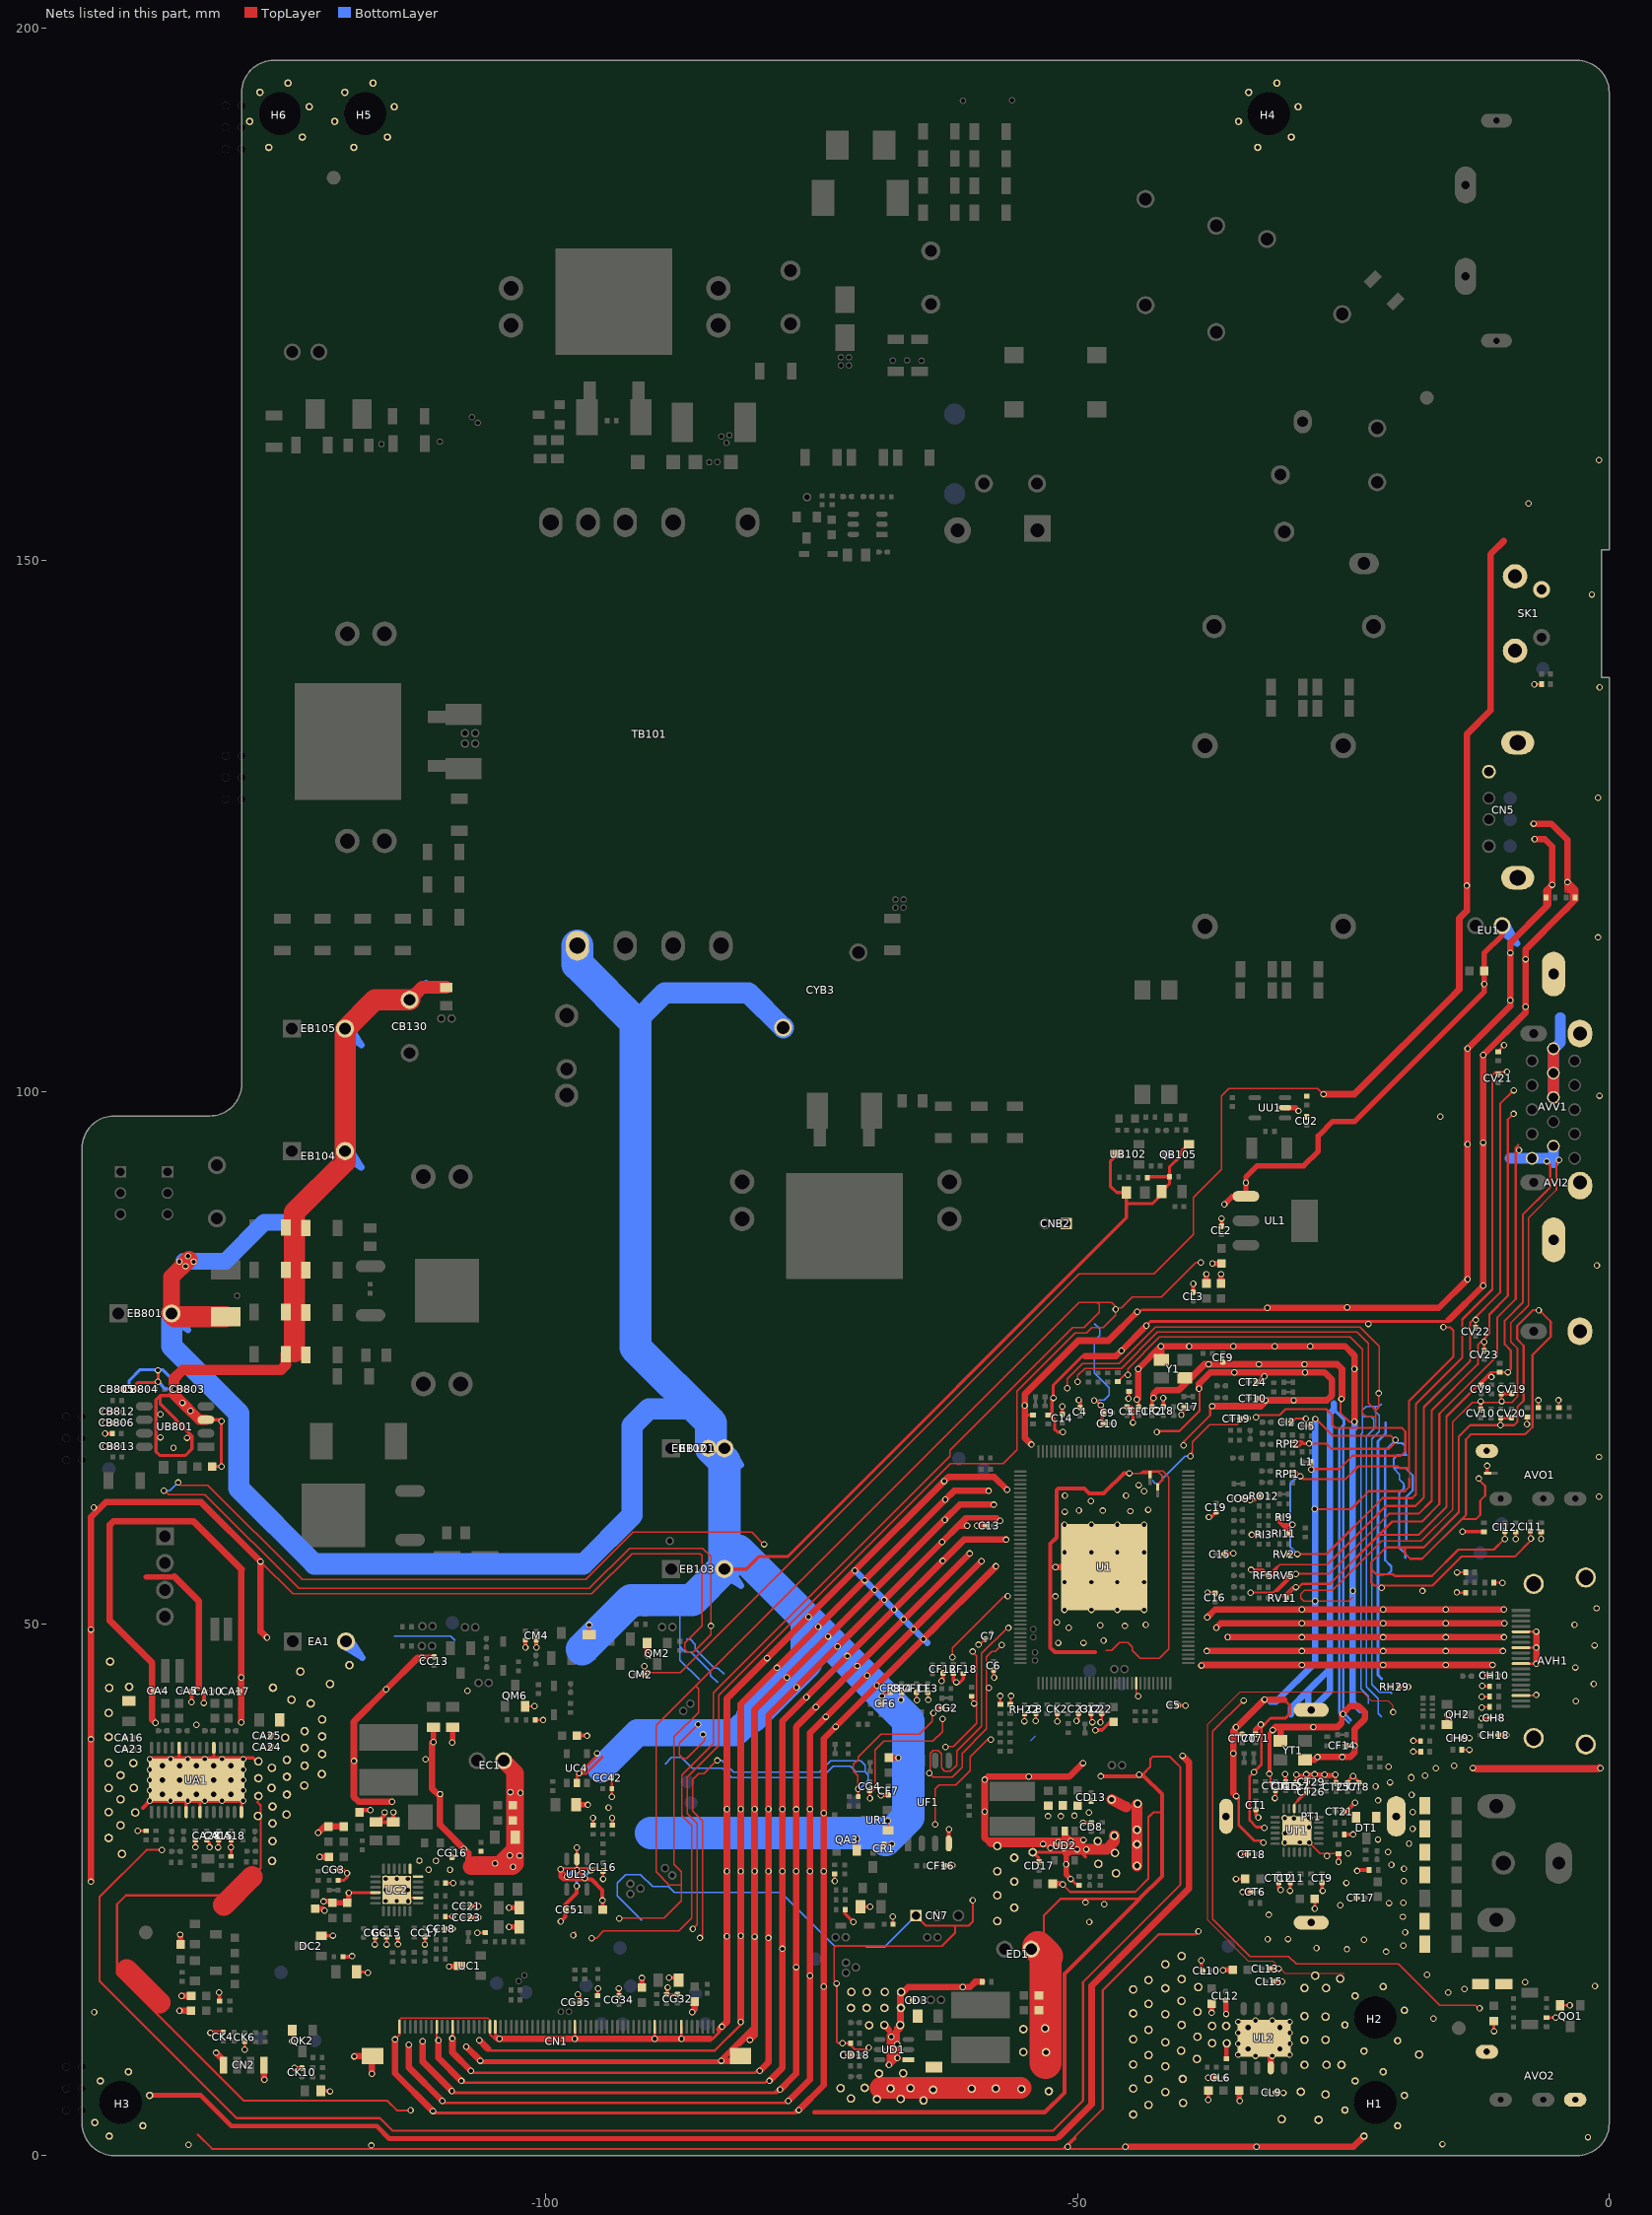
[diagram p0: the nets of this part, all layers, seen from the top]
# Altium PCB MISC86383-9.PcbDoc (part 10 of 18)
Units mm, origin at the board's own origin, x right, y up, seen from the top; angles counter-clockwise.
Board outline 143.6 x 197 mm, 2 copper layers (TopLayer, BottomLayer), stack 1.571 mm thick; 743 components, 401 nets, 2996 pads, 1077 vias.
Unrouted connection lines stored in the file: 4.

## Via types
v1: diameter 0.6, hole 0.4, TopLayer to BottomLayer, tented both sides, 993 vias
v2: diameter 0.6, hole 0.4, TopLayer to BottomLayer, 65 vias
v3: diameter 0.7, hole 0.5, TopLayer to BottomLayer, tented both sides, 15 vias
v4: diameter 0.8, hole 0.5, TopLayer to BottomLayer, tented both sides, 4 vias

## Nets (pads, with @x,y where several pads share a name; then routed paths per layer and width w, separated by ;. In a path a pad name is that pad's centre, name@x,y a point inside that pad or via, vN(x,y) a via of type N, cw(c..) or ccw(c..) an arc to the next point about the centre after c; other vN are vias at no path point) (continued)
GND: (continued)
  TopLayer w0.203: v1(-138.372,30.534) RA1.1@-137.578,30.534 ; v1(-136.105,28.735) -137.55,28.735 -141.962,24.323 -141.962,16.383 -129.084,3.505 ; RA14.1@-132.947,29.659 -132.947,29.053 -132.939,29.046 v1(-132.939,28.981) ; -132.715,1.956 -131.386,0.627 -51.386,0.627 ; -128.321,3.505 -129.084,3.505 ; CK6.1@-128.321,10.7 -128.321,9.97 v1(-128.308,9.957) ; -127.114,33.223 -126.809,32.918 -126.809,27.026 -129.375,24.46 -139.49,24.46 -140.311,23.639 -140.311,17.067 -128.4,5.156 -114.912,5.156 -113.998,4.242 v1(-112.712,4.242) ; v1(-114.173,10.909) -113.75,11.332 CN1.1@-113.75,12.103 ; CN1.8@-110.25,12.103 -110.25,10.987 v1(-110.084,10.82) ; v1@-108.75,10.808 CN1.11@-108.75,12.103 ; v1(-106.426,20.93) -106.426,20.98 -106.394,20.948 RC3.1@-105.715,20.948 ; CN1.18@-105.25,12.103 -105.25,11.398 -104.825,10.973 ; CN1.19@-104.75,12.103 -104.75,11.38 v1(-104.343,10.973) ; QM6.E@-101.943,42.228 -101.105,42.228 v1(-101.067,42.266) ; RM10.2@-100.997,40.957 -100.266,40.957 v1(-100.254,40.945) ; v1(-97.422,20.697) -97.235,20.884 -97.235,20.996 ; v1(-97.282,10.973) -97.25,11.005 CN1.34@-97.25,12.103 ; RG12.1@-95.123,15.024 -95.123,15.672 -95.098,15.697 v1(-95.098,15.71) ; v1(-89.764,10.973) -89.75,10.986 CN1.49@-89.75,12.103 ; CN1.54@-87.25,12.103 -87.25,10.987 v1(-87.236,10.973) ; RA38.1@-72.83,26.484 -72.83,25.87 -72.819,25.859 v1(-72.819,25.807) ; v1(-72.649,16.186) -72.644,16.181 -72.644,10.693 -72.517,10.566 v1(-72.085,10.566) -72.079,10.56 RD5.1@-71.343,10.56 -71.343,10.383 -70.942,9.982 -69.748,9.982 -69.596,10.135 v1(-69.621,10.135) ; v1(-72.034,9.449) -72.009,9.449 -72.007,9.451 CD18.1@-71.345,9.451 ; QA3.E@-70.744,28.713 -70.744,29.767 v1(-70.731,29.78) ; v1(-70.637,34.468) -70.637,34.315 -70.619,34.297 RR2.2@-70.619,33.757 ; CG4.2@-69.545,34.297 -69.545,33.63 v1(-69.52,33.604) ; CF6.2@-68.472,42.469 -68.472,43.11 v1(-68.377,43.205) -68.065,43.517 CF8.2@-67.615,43.517 ; CR1.1@-68.191,29.291 -68.184,29.298 v1(-67.454,29.298) ; v1(-67.835,31.457) -67.81,31.431 UR1.1@-67.81,30.58 ; v1(-67.359,22.456) -67.359,22.413 -67.334,22.388 RA31.1@-67.334,21.754 ; v1(-66.598,42.839) -66.562,42.875 -66.548,42.875 CF4.2@-66.548,43.517 ; CN7.1@-65.195,22.555 -64.255,21.615 -61.493,21.615 ; CF11.2@-65.151,43.517 -65.151,42.875 v1(-65.1,42.824) ; CF3.2@-64.069,43.521 -64.069,43.008 -64.042,42.981 v1(-64.042,42.844) ; v1@-63.599,41.607 -63.094,42.113 CG2.2@-62.782,42.113 ; -62.743,19.71 -61.493,20.96 -61.493,21.615 ; DR1.A@-59.957,43.187 -59.957,42.939 -59.703,42.685 -59.703,42.52 v1(-59.715,42.507) ; v1(-59.842,24.003) -59.842,21.996 -60.223,21.615 -61.493,21.615 ; v1(-59.294,48.036) -59.396,48.137 -59.091,48.137 C7.1@-58.68,48.548 ; DV2.A@-57.262,42.415 v1(-57.262,43.21) ; DV1.A@-56.297,42.415 -56.297,43.159 v1(-56.246,43.21) ; v1(-54.988,40.837) -54.988,40.899 -54.976,40.912 RH22.1@-54.976,41.515 ; ED1.2@-54.351,19.406 -53.162,20.594 -53.162,22.552 -51.585,24.13 -44.181,24.13 -44.162,24.149 ; v1(-53.934,40.875) -53.91,40.9 -53.91,41.002 C8.1@-53.91,41.553 C8.1@-53.91,41.728 ; v1(-51.903,40.835) CK2.2@-51.903,41.553 ; v1(-51.384,25.476) -50.698,24.79 -44.581,24.79 -43.332,26.039 -43.332,31.801 -42.875,32.258 -42.056,32.258 ; v1@-51.013,0.789 v1@-50.981,0.821 ; v1(-50.911,0.821) v1@-50.981,0.821 ; DT3.A@-46.215,72.765 -45.587,73.393 v1(-45.263,73.393) ; v1(-45.494,0.826) -45.693,0.627 -51.386,0.627 ; v1@-44.226,35.839 v1(-44.194,35.808) ; -44.028,64.152 -43.86,64.321 -43.307,64.321 -42.443,64.321 -42.021,63.899 -42.021,63.516 -42.021,63.482 RA2.JP_2K@-42.456,63.047 ; -43.891,35.801 -43.147,36.545 -43.147,37.281 -42.933,37.495 -41.305,37.495 -40.594,36.784 ; v1(-42.543,68.038) -42.467,68.114 -40.421,68.114 -38.521,70.014 ; -40.967,37.158 -40.316,36.507 -40.316,25.469 -49.484,16.301 -49.484,5.15 -52.306,2.329 -114.42,2.329 -115.596,3.505 -129.084,3.505 ; v1(-40.029,66.781) -40.029,67.105 -37.53,69.604 -37.53,70.256 v1(-37.327,70.459) ; v1(-38.618,21.078) -38.893,20.803 -42.36,20.803 -47.63,15.533 -47.63,4.382 -50.228,1.784 ; v1(-38.568,72.115) -38.521,72.068 -38.521,70.014 ; -38.521,70.663 -38.521,70.014 ; CT19.1@-34.66,69.27 -34.601,69.329 v1(-33.982,69.329) ; v1(-33.733,52.928) -33.713,52.948 -31.587,52.948 -31.461,53.075 ; v1(-33.225,69.408) v1@-33.182,69.366 ; v1@-33.182,69.291 v1@-33.182,69.366 ; v2(-31.953,35.89) -31.858,35.795 -31.858,34.79 CT14.1@-31.379,34.311 ; -30.687,52.547 -29.791,53.444 v1(-29.462,53.444) v1@-29.498,53.407 ; RV11.1@-30.342,52.428 -30.342,52.564 v1@-29.498,53.407 ; RV5.1@-30.139,54.562 -30.139,54.397 -31.461,53.075 ; RV5.1@-30.136,54.683 -29.733,54.683 v1@-29.661,54.611 ; RV2.1@-30.136,56.512 -29.444,56.512 -29.307,56.649 v1(-29.307,56.552) -26.563,56.552 -21.305,61.811 ; CI2.1@-29.856,68.963 -29.517,69.302 v1@-28.53,69.302 ; RPI1.6@-29.797,63.849 -29.074,63.849 v1(-29.053,63.871) -28.794,63.612 -24.79,63.612 -23.594,64.808 -19.875,64.808 -19.71,64.643 -18.877,64.643 -18.826,64.694 ; v1@-29.589,53.407 v1@-29.498,53.407 ; v1@-29.447,54.689 -26.351,54.689 -20.697,60.343 -17.909,60.343 -16.698,61.554 -16.698,70.058 -12.344,74.411 -12.344,76.238 -11.273,77.309 -11.273,79.083 -9.522,80.834 -9.522,97.418 v1(-8.992,97.949) v1@-8.9,98.04 ; v1@-28.591,69.2 v1(-28.51,69.282) ; v1(-28.227,66.944) -26.6,66.944 -26.114,66.458 -20.714,66.458 -20.01,67.162 v1@-20.01,67.276 ; L1.1@-28.018,65.23 -28.024,65.224 v1@-28.024,64.544 ; CI5.1@-27.908,68.709 CI5.1@-28.022,68.595 -28.022,68.868 v1(-27.634,69.256) -27.546,69.256 -25.96,67.67 -20.502,67.67 -20.108,67.276 v1@-20.01,67.276 ; v1(-27.683,60.793) -27.683,60.78 -24.285,60.78 -22.594,62.471 -19.202,62.471 -18.801,62.873 -18.801,63.628 ; -26.426,55.652 -21.001,61.077 -18.213,61.077 -17.432,61.858 -17.432,70.362 ; -25.253,68.415 -25.753,68.415 ; v1(-25.179,71.15) -25.277,71.051 -25.277,69.833 -24.434,68.991 v1(-23.96,68.991) ; v1(-21.395,53.382) v1@-21.187,53.59 ; -20.939,61.811 -21.305,61.811 ; v1(-20.087,67.276) v1@-20.01,67.276 ; v1@-19.96,67.276 v1@-20.01,67.276 ; RH29.2@-19.769,44.061 -18.925,44.061 v1(-18.909,44.077) ; -19.703,58.356 -21.641,58.356 -21.643,58.359 ; -19.702,58.357 -17.923,58.357 -15.303,60.977 -15.303,69.48 -11.128,73.655 DI2.A@-10.274,73.655 v1(-9.522,73.655) -9.251,73.925 -9.251,75.701 -9.821,76.271 -9.821,78.507 -8.128,80.2 -8.128,88.465 -5.55,91.043 -5.55,93.161 v1(-5.88,93.491) ; -19.218,57.186 -20.971,57.186 -22.377,55.78 -22.377,55.143 ; -18.826,64.265 -18.826,64.694 ; -18.53,71.235 -18.826,70.939 ; v1(-18.419,37.976) -18.419,37.954 -17.717,37.954 DV8.A@-17.715,37.952 ; v1(-18.408,38.995) -18.303,38.995 -18.278,38.969 DV7.A@-17.731,38.969 ; -17.962,70.87 -18.166,70.666 ; -17.143,70.65 -17.432,70.362 ; v1(-15.583,77.889) -14.973,77.889 -14.648,77.564 -14.648,75.117 -18.826,70.939 ; v1(-14.326,52.946) -14.296,52.916 DH2.A@-13.499,52.916 ; v1(-14.313,54.839) -14.305,54.847 DV4.A@-13.499,54.847 ; DK2.A@-13.85,38.151 -13.259,38.151 v1(-13.157,38.151) ; -13.729,56.972 -14.18,56.972 ; CV22.1@-12.56,77.895 -12.56,78.537 -12.548,78.549 -12.548,78.566 v1(-12.541,78.572) ; v1(-12.26,63.652) -12.355,63.652 -11.652,62.95 -11.652,62.038 -12.116,61.575 -12.116,60.249 -12.528,59.836 -13.857,59.836 ; v1(-11.989,41.115) CH8.1@-11.246,41.115 ; v1(-11.989,42.131) -11.989,42.233 -11.939,42.182 DH7.A@-11.246,42.182 ; v1(-11.989,43.147) DH6.A@-11.246,43.147 ; v1(-11.939,44.163) -11.888,44.163 -11.837,44.112 DH3.A@-11.246,44.112 ; CV23.1@-11.747,75.71 v1(-11.747,76.505) ; DV3.A@-10.835,53.861 -10.046,53.861 v1(-10.033,53.848) ; DI3.A@-10.439,103.79 -10.439,103.861 v1(-9.881,104.419) ; CI12.2@-9.804,58.655 v1(-9.804,57.963) -9.858,57.963 -10.849,56.972 -14.18,56.972 ; v1(-9.601,101.892) -10.668,101.892 -10.991,101.57 -10.991,81.442 -13.813,78.62 -13.813,75.019 -18.166,70.666 ; v1(-8.982,100.165) -10.257,98.89 -10.257,81.138 -13.078,78.316 -13.078,74.715 -17.432,70.362 ; v1(-8.788,57.963) -8.788,58.064 DO1.A@-8.788,58.655 ; -8.547,95.021 -8.788,94.78 -8.788,94.247 ; v1(-8.484,94.551) -8.788,94.247 ; AVH1.17@-8.3,43.25 -7.042,43.25 -6.985,43.307 v1(-6.858,43.307) ; AVH1.11@-8.3,46.25 -7.007,46.25 -6.985,46.228 v1(-6.858,46.228) ; AVH1.8@-8.3,47.75 -7.114,47.75 -7.112,47.752 v1(-6.858,47.752) ; AVH1.5@-8.3,49.25 -7.011,49.25 -6.985,49.276 v1(-6.858,49.276) ; CI11.2@-7.417,58.706 -7.417,58.014 v1(-7.366,58.014) -7.366,57.839 -8.893,56.312 -13.906,56.312 -16.628,53.59 v1@-21.187,53.59 ; v1(-7.046,138.326) -6.96,138.326 -6.932,138.354 DK1.A@-6.369,138.354 ; DV6.A@-6.655,70.326 -6.655,70.95 v1(-6.655,71.018) ; v1@-6.401,57.963 DO3.A@-6.401,58.655 ; DI5.A@-5.893,12.968 -5.043,12.968 v1(-5.029,12.954) ; v1(-4.775,71.018) -4.775,70.968 -4.724,70.917 DV5.A@-4.724,70.326 ; QO1.E@-4.61,14.118 -3.815,14.118 -3.81,14.122 v1(-3.708,14.122) ; -51.386,0.627 -50.228,1.784 ; v1@-50.981,0.821 -50.228,1.574 -50.228,1.784 ; v1@-33.182,69.366 -32.927,69.621 -30.996,69.621 -30.441,70.177 -26.609,70.177 -26.038,69.606 -26.038,68.7 -25.753,68.415 ; -31.461,53.075 -31.198,53.075 v1@-29.661,54.611 ; v1@-29.661,54.611 -29.596,54.676 v1(-29.458,54.676) -29.561,54.574 -29.561,54.511 v1@-29.661,54.611 ; v1@-29.498,53.407 -29.218,53.407 -28.881,53.744 -26.258,53.744 -21.643,58.359 ; v1@-28.024,64.544 -28.018,64.55 -25.376,64.55 -24.127,65.798 -19.598,65.798 -19.164,66.232 -19.164,68.086 -19.493,68.415 -22.081,68.415 -25.753,68.415 ; v1@-28.024,64.544 v1(-28.024,64.518) -27.999,64.544 v1@-28.024,64.544 ; -22.377,55.143 -22.377,53.87 -22.098,53.59 v1@-21.187,53.59 ; -22.377,55.143 -21.891,54.657 -20.342,54.657 -20.172,54.487 -16.665,54.487 -14.18,56.972 ; -21.643,58.359 -20.393,59.609 -17.605,59.609 -15.964,61.25 -15.964,69.754 -10.539,75.178 -10.539,78.779 -8.788,80.53 -8.788,94.247 ; -21.305,61.811 -18.517,61.811 -18.166,62.162 -18.166,70.666 ; -18.826,64.694 -18.826,70.939 ; -13.857,59.836 -17.581,56.113 -18.719,56.113 -19.218,56.612 -19.218,57.189 -17.439,57.189 -14.135,60.493 -14.135,67.615 -13.077,68.672 -8.937,68.672 -8.639,68.971 -8.639,70.387 -8.047,70.979 -8.047,76.149 -8.653,76.755 -8.653,78.023 -7.19,79.486 v1(-6.629,79.486) -6.568,79.486 -5.502,78.42 -5.502,76.986 -7.213,75.275 -7.213,68.491 -7.894,67.811 -13.005,67.811 -13.474,67.341 -13.474,60.219 -13.857,59.836
  TopLayer w0.229: -84.11,9.863 -81.668,12.305 v1(-81.668,12.548) ; v1(-50.1,40.86) -50.1,40.898 -49.909,41.089 C23.1@-49.909,41.54 ; C12.1@-48.677,41.553 -48.677,40.822 v1(-48.601,40.746) ; v1(-47.839,40.72) -47.725,40.835 C22.1@-47.725,41.553
  TopLayer w0.254: v1(-118.516,24.701) -118.495,24.723 UC2.4@-116.014,24.723 ; v1(-116.075,19.845) -116.075,19.947 -116.046,19.975 CG6.2@-116.046,20.53 ; CC15.2@-114.98,20.53 -114.98,19.982 -114.97,19.972 v1(-114.97,19.845) ; UC2.25@-114.014,24.973 -113.264,24.223 UC2.14@-112.014,24.223 ; RG14.1@-113.925,20.53 -113.919,20.524 -113.919,19.875 -113.913,19.869 v1(-113.913,19.853) ; v1(-111.376,19.845) -111.376,19.959 -111.36,19.975 CC17.1@-111.36,20.53 ; -111.125,4.674 -110.457,4.005 -76.722,4.005 ; -110.426,5.639 -109.738,4.95 -77.616,4.95 -77.587,4.978 ; v1(-110.084,10.82) -110.033,10.82 -110.033,9.866 ; CC18.1@-109.459,21.302 -108.844,21.302 -108.826,21.32 v1(-108.775,21.32) ; RC12.1@-109.459,22.471 -108.907,22.471 -108.89,22.488 v1(-108.775,22.488) ; RG13.1@-109.414,25.618 -108.882,25.618 -108.877,25.613 v1(-108.725,25.613) ; -109.169,6.274 -108.79,5.895 -78.51,5.895 ; v1@-107.761,6.84 -79.404,6.84 -79.036,7.208 v1@-78.785,7.208 ; v1(-107.044,7.962) -106.867,7.785 -80.299,7.785 -79.677,8.407 -79.425,8.407 ; CC23.1@-107.019,22.396 -106.394,22.396 -106.375,22.377 v1(-106.337,22.377) ; CC21.2@-107.018,23.463 -106.407,23.463 -106.375,23.431 v1(-106.337,23.431) ; v1@-105.897,8.905 -83.75,8.905 -80.545,12.11 -80.545,12.319 -80.368,12.497 ; -105.432,10.028 -105.254,9.85 -84.141,9.85 ; v1(-97.996,26.227) -97.996,26.295 v1(-98.606,26.904) -98.494,27.015 v1@-97.079,27.015 ; v1(-97.079,28.943) -97.079,28.842 UL3.2@-97.079,27.879 v1@-97.079,27.015 ; UC4.2@-97.079,35.036 -97.079,35.725 v1(-96.863,35.941) v1@-96.83,35.941 ; v1(-96.343,26.085) -96.343,26.098 v1(-97.068,26.823) -97.079,26.833 v1@-97.079,27.015 ; v1(-95.567,31.737) -95.567,31.712 -95.555,31.699 RL3.1@-95.555,31.057 ; -95.282,27.015 v1@-97.079,27.015 ; v1(-95.173,37.826) -95.173,37.598 v1@-96.83,35.941 ; -94.693,37.453 -96.205,35.941 v1@-96.83,35.941 ; CL16.2@-94.615,26.689 -94.615,26.213 -94.602,26.2 v1(-94.602,26.01) ; v1(-94.092,32.711) -94.07,32.689 v1@-94.07,32.62 ; RC35.2@-93.783,34.493 v1(-93.783,33.738) CC42.2@-93.783,35.496 ; v1(-93.764,31.737) -93.726,31.699 RL7.1@-93.726,31.057 ; -84.319,10.973 -82.969,12.323 -82.969,12.574 ; v1(-77.967,6.187) -78.259,5.895 -78.51,5.895 ; -77.661,6.744 -78.51,5.895 ; v1(-77.198,5.123) -77.198,5.063 -77.282,4.978 -77.587,4.978 ; -77.072,5.494 -77.587,4.978 ; C6.1@-57.891,45.622 -57.891,45.043 -57.937,44.997 -57.893,44.997 v1(-57.841,44.945) ; v1(-52.273,71.24) -52.273,72.431 -49.542,75.163 -49.398,75.163 ; v1(-50.648,26.01) -50.033,25.395 RD8.2@-49.851,25.395 ; v1(-49.475,31.297) -49.458,31.314 CD8.1@-48.701,31.314 ; -44.503,78.951 -43.927,79.527 -16.188,79.527 ; v1@-44.497,71.103 v1@-44.425,71.031 ; v1(-44.425,71.082) v1@-44.425,71.031 ; CF1.1@-44.249,70.402 -44.249,70.855 v1@-44.425,71.031 ; v1(-43.525,78.029) -43.129,78.425 -22.888,78.425 ; v1@-35.138,33.855 v1(-35.079,33.797) -34.846,33.564 -34.846,31.087 -33.365,29.606 -32.687,29.606 v1(-32.509,29.428) ; -35.138,39.66 -35.108,39.629 CT70.2@-34.52,39.629 ; v1(-34.457,24.767) CT6.2@-33.714,24.767 ; v1(-33.612,58.372) -33.459,58.372 RI3.1@-32.907,58.372 ; v1@-32.699,40.287 v1@-32.699,40.254 ; v1(-32.412,30.82) -32.481,30.888 -33.175,30.888 -33.805,31.518 -33.805,35.649 v1(-33.394,36.06) -32.699,36.755 v1@-32.699,40.254 ; CL9.1@-31.325,5.944 -30.785,5.944 -30.734,5.893 v1(-30.632,5.893) ; -30.574,42.878 -30.025,42.328 -30.025,41.531 -30.429,41.127 -31.826,41.127 v1@-32.699,40.254 ; RPI2.6@-29.771,66.656 -29.741,66.686 -29.184,66.686 -28.824,67.046 ; RPI2.4@-29.771,67.156 -29.767,67.151 -28.93,67.151 -28.824,67.046 ; v1(-28.227,66.944) -28.723,66.944 -28.824,67.046 ; v1(-22.657,78.194) -22.888,78.425 ; -15.076,78.577 -15.229,78.425 -22.888,78.425 ; v1(-11.925,45.136) -11.913,45.148 CH10.1@-11.245,45.148 ; CO77.2@-10.846,12.659 -10.846,11.709 v1(-10.82,11.684) ; CH18.1@-10.371,39.54 v1(-9.678,39.54) ; -76.722,4.005 -76.455,4.271 v1(-76.204,4.271) -76.47,4.005 -76.722,4.005
  TopLayer w0.3: v2(-141.465,69.952) CB812.1@-140.766,69.952 ; v2(-141.453,67.894) RB803.1@-140.77,67.894 ; v2(-141.453,68.885) CB806.2@-140.77,68.885 ; v2(-141.427,66.675) CB813.1@-140.569,66.675 ; CB805.1@-139.885,72.047 v2(-139.179,72.047) -139.167,72.06 CB804.2@-138.5,72.06 -138.5,72.574 -138.392,72.682 -136.525,72.682 v2(-136.461,72.746) v2(-136.461,73.838) ; -134.975,71.576 -135.088,71.463 -136.258,71.463 ; v2(-134.901,72.074) CB803.2@-134.162,72.074 ; UB801.3@-131.961,69.18 -130.635,69.18 v2(-130.505,69.05) v2(-130.505,64.795) CB801.1@-131.361,64.795 ; UB102.A@-46.203,94.171 -46.914,93.46 -46.914,91.161 -46.304,90.551 RB181.1@-45.392,90.551 -45.392,89.535 -45.367,89.51 -42.926,89.51 -42.089,90.347 CB115.2@-42.089,90.627 -41.344,91.371 RB183.2@-41.344,92.024 ; RB134.1@-43.441,91.948 -43.365,92.024 RB183.2@-41.344,92.024 ; QB105.E@-39.522,95.085 -39.56,95.085 -40.31,94.336 -40.31,93.998 -41.344,92.963 RB183.2@-41.344,92.024 ; -136.258,71.463 -136.659,71.062 -136.659,66.187 -136.296,65.824 -133.896,65.824 -133.274,66.446 -133.274,67.665 -136.258,70.649 -136.258,71.463
  TopLayer w0.305: v1(-137.238,37.27) -137.109,37.399 -134.47,37.399 ; UA1.24@-134.47,38.341 -134.47,37.399 ; UA1.6@-133.82,32.291 -133.82,33.362 -133.82,34.341 v3(-132.845,35.316) ; UA1.8@-132.52,32.291 -132.52,33.362 -132.52,34.991 v3(-132.845,35.316) ; CA28.1@-131.88,29.659 -131.637,29.416 -131.637,29.006 -131.623,28.992 v1(-131.623,28.981) ; UA1.19@-131.22,38.341 -131.22,37.399 ; v1(-130.81,28.972) -130.757,28.972 -130.762,28.977 CA15.2@-130.762,29.658 ; v1(-130.734,15.316) -130.683,15.265 RC27.1@-130.683,14.522 ; v1(-129.601,28.981) -129.601,29.002 v1@-129.598,29.006 ; RA12.2@-129.598,28.121 v1@-129.598,29.006 ; CA18.2@-129.594,29.658 -129.594,29.01 v1@-129.598,29.006 ; UA1.14@-128.62,32.291 -128.62,33.194 v1(-128.452,33.362) ; pad.VIA5@-127.036,37.052 -127.189,37.052 -127.536,37.399 -128.969,37.399 -129.555,37.399 -131.22,37.399 ; v1(-123.85,10.757) -123.838,10.77 QK2.E@-123.838,11.786 ; v1(-123.647,8.242) -123.558,8.242 -123.553,8.248 CK10.1@-122.936,8.248 ; DK20.K@-121.156,6.094 -120.343,6.094 v1(-120.282,6.032) ; DC2.3@-121.101,20.657 -120.034,20.657 v1(-120.015,20.676) ; CG3.2@-119.532,26.878 -119.029,26.878 v1(-118.694,26.543) -118.694,26.187 -119.007,25.875 RG16.1@-119.528,25.875 ; CC30.2@-117.804,17.259 -116.815,17.259 v1(-116.738,17.183) ; v1(-96.977,15.138) -96.977,15.088 -96.743,14.853 CG35.2@-96.743,14.402 ; CM5.1@-95.936,48.985 -95.936,49.797 -95.92,49.813 v1(-95.92,49.887) ; v1(-93.142,15.723) -93.104,15.684 -93.104,15.583 -93.116,15.57 CG34.1@-93.116,15.043 ; v1(-90.716,46.025) -90.697,46.006 CM2.2@-90.697,45.212 ; v1(-88.532,15.811) -88.532,15.748 -88.595,15.684 -88.595,15.17 RG44.1@-88.633,15.132 -87.655,15.132 CG32.1@-87.617,15.17 ; v1(-88.405,16.726) -87.808,16.726 -87.566,16.485 CC29.2@-87.502,16.485 ; EB103.2@-83.212,55.143 -81.135,55.143 -79.957,56.321 -77.264,56.321 -45.392,88.193 -45.392,89.535 ; RA18.1@-71.855,23.125 -71.855,22.757 v1(-71.069,21.971) ; CA36.1@-70.414,23.398 -69.543,23.398 -69.537,23.405 v1(-69.512,23.405) ; v1(-68.486,33.858) -68.377,33.858 -68.364,33.871 CF7.2@-67.783,33.871 ; v1@-62.776,44.602 v1(-62.776,44.615) -62.649,44.742 CF12.2@-62.649,45.32 ; RF13.2@-61.665,45.31 -61.665,44.609 v1@-61.468,44.412 ; v1(-61.379,44.501) v1@-61.468,44.412 ; RF18.2@-60.754,45.318 -60.754,44.793 -61.135,44.412 v1@-61.468,44.412 ; v1(-59.446,59.212) C13.1@-58.703,59.212 ; -54.966,69.716 -54.883,69.633 DU1.A@-54.204,69.633 ; CD17.1@-53.619,27.654 -53.619,27.92 pad.VIA5@-54.216,28.516 -50.959,28.516 -49.682,28.516 -49.233,28.066 ; DU2.A@-52.73,69.633 -52.552,69.633 -52.148,69.229 -52.148,68.302 -51.867,68.021 v1(-51.384,68.021) ; -52.402,69.633 -52.402,71.111 v1(-52.273,71.24) ; C14.1@-51.435,69.735 -51.435,70.307 v1(-51.435,70.434) ; v1(-49.875,71.033) -49.739,71.033 -49.714,71.008 -49.714,70.398 C4.1@-49.757,70.355 ; v1(-48.436,70.989) -48.237,70.989 v1(-47.801,70.553) -47.661,70.413 -47.661,68.988 C10.1@-47.59,68.917 ; C11.1@-46.607,40.763 -46.943,40.763 -47.684,40.022 ; C3.1@-45.337,70.419 -44.974,70.419 -44.78,70.225 v1(-44.78,68.923) ; v1(-45.199,71.183) -45.199,71.26 -45.149,71.31 DT2.A@-45.149,71.863 ; CF2.1@-42.979,70.414 -42.979,71.082 v1(-42.848,71.213) ; v1(-41.946,71.213) -41.912,71.179 C18.1@-41.912,70.427 ; C5.1@-40.531,42.333 -39.876,42.333 v1(-39.851,42.308) ; v1(-40.234,69.659) -40.234,69.799 -40.011,70.022 C17.1@-40.011,70.371 ; v1(-38.35,18.339) -38.35,17.453 CL10.1@-38.271,17.374 ; v1(-37.77,52.908) -37.77,52.895 -37.744,52.87 -37.713,52.901 C16.1@-37.059,52.901 ; v1(-37.643,60.033) -37.643,59.982 -37.472,59.982 C19.1@-36.944,60.51 ; C15.1@-36.151,56.54 -36.062,56.629 v1(-35.344,56.629) ; v1(-35.092,26.012) CT5.1@-34.224,26.012 ; v1(-34.744,28.361) -34.706,28.323 CT18.1@-34.039,28.323 ; CO9.1@-34.457,61.889 -34.453,61.889 -34.174,61.61 v1(-33.777,61.61) -33.288,61.61 RO12.2@-32.907,61.991 ; v1(-33.678,55.076) -33.668,55.066 -32.573,55.066 RF5.2@-32.069,54.562 RF5.2@-31.986,54.562 ; CT1.1@-33.225,32.508 -33.225,32.019 v1(-32.996,31.79) ; CT10.2@-33.096,71.184 -32.512,71.184 v1(-32.343,71.015) ; CT24.1@-33.096,72.721 -32.564,73.254 v1(-32.41,73.254) ; v1(-31.43,33.606) -31.379,33.657 CT14.1@-31.379,34.311 ; -31.35,55.142 -31.544,54.948 -31.544,54.8 -31.782,54.562 RF5.2@-31.986,54.562 ; -31.275,55.273 RF5.2@-31.986,54.562 ; CT12.2@-31.067,25.637 -31.067,25.116 v1@-30.915,24.963 ; v1@-30.915,24.976 v1@-30.915,24.963 ; v1(-30.909,24.958) v1@-30.915,24.963 ; v1(-30.465,35.867) -30.439,35.841 -30.439,35.161 CT15.1@-30.414,35.135 ; v1@-29.987,24.914 CT11.1@-29.987,25.638 ; CT27.2@-29.436,35.123 -29.436,35.765 v1(-29.398,35.803) ; -29.252,33.397 -29.252,33.402 CT26.1@-28.451,34.203 CT29.1@-28.451,35.13 ; CT2.1@-27.68,24.132 -27.675,24.127 v1(-27.675,23.218) ; CT9.2@-26.997,25.637 -26.997,24.953 v1(-26.939,24.894) ; v1(-25.753,35.803) -25.727,35.778 CT25.2@-25.727,35.073 ; CT7.1@-24.597,35.073 -24.597,35.155 v1(-24.076,35.676) -23.53,35.131 CT8.1@-23.53,35.073 ; QH2.E@-15.241,40.518 v1(-15.241,41.445) ; CH9.1@-13.851,39.261 v1(-13.132,39.261) ; v1(-13.805,58.674) -13.786,58.655 DO2.A@-11.786,58.655 ; v1(-12.827,36.436) -12.573,36.182 -0.978,36.182 -0.749,36.411 v1(-0.826,36.411) ; v1(-12.09,70.917) -12.084,70.911 -12.084,70.819 -12.084,70.813 CV10.1@-12.084,70.2 ; CV9.1@-12.032,72.481 -12.032,72.6 -11.43,73.203 v1(-11.074,73.203) ; v1(-11.468,64.859) -11.468,64.196 RI10.JP_1K@-11.432,64.16 ; v1(-10.211,68.672) -10.211,68.783 -10.205,68.789 RV14.2@-10.205,69.35 CV20.1@-9.246,69.35 ; v1(-10.109,70.917) -10.153,70.96 RV4.2@-10.153,71.631 -9.224,71.631 CV19.1@-9.195,71.66 ; -134.47,37.399 -131.22,37.399 ; -134.47,37.399 -134.47,36.941 v3(-132.845,35.316) ; v3(-132.845,35.316) -131.22,36.941 -131.22,37.399 ; -47.684,40.022 -48.271,40.022 v1(-48.309,39.984) -47.722,39.984 -47.684,40.022